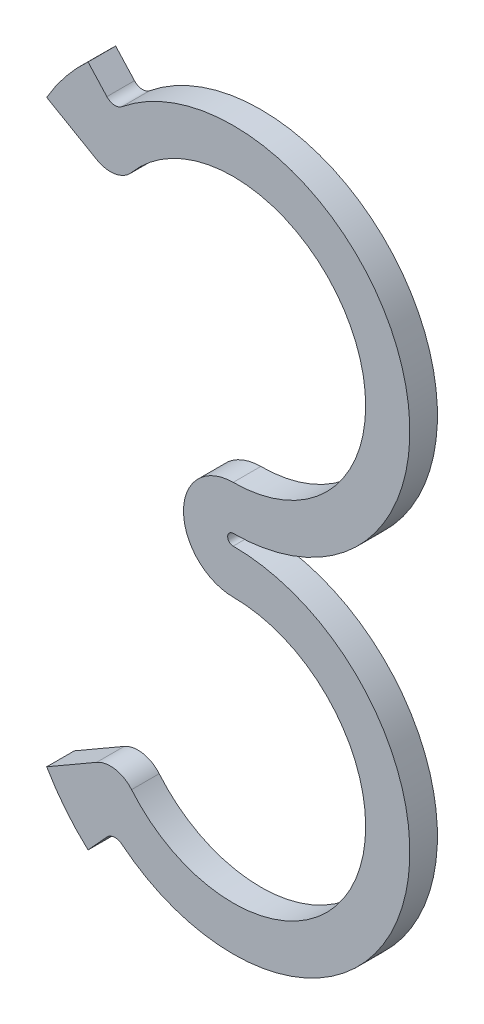
from build123d import *

# Parameters (mm, degrees)
EXTRUDE_1_DEPTH        = 2.5
FILLET_1_R             = 1
FILLET_2_R             = 2.5
FILLET_1_OF_MIRROR_1_R = 1
FILLET_2_OF_MIRROR_1_R = 2.5


with BuildPart() as part:
    # 草图2 → 凸台-拉伸1 (new body)
    with BuildSketch(Plane.XY):
        with BuildLine():
            Line((-4.5, -6.579113924), (-0.5, -6.579113924))
            ThreePointArc((-0.5, -6.579113924), (-0.353553391, -6.225560533), (0, -6.079113924))
            ThreePointArc((0, -6.079113924), (14.918190439, 15.70427557), (-10.784713231, 21.739936821))
            Line((-10.784713231, 21.739936821), (-13.143869251, 24.325354172))
            ThreePointArc((-13.143869251, 24.325354172), (-15.194957506, 22.142312604), (-16.887495374, 19.670886076))
            Line((-16.887495374, 19.670886076), (-10.392304845, 15.920886076))
            ThreePointArc((-10.392304845, 15.920886076), (10.392304845, 15.920886076), (0, -2.079113924))
            ThreePointArc((0, -2.079113924), (-3.181980515, -3.397133409), (-4.5, -6.579113924))
        make_face()
    extrude_1 = extrude(amount=EXTRUDE_1_DEPTH)

    # 圆角1
    fillet_1_edges = [part.edges().sort_by_distance(p)[0] for p in [
        (-10.784713231, 21.739936821, 1.25),
    ]]
    fillet(fillet_1_edges, radius=FILLET_1_R)

    # 圆角2
    fillet_2_edges = [part.edges().sort_by_distance(p)[0] for p in [
        (-10.392304845, 15.920886076, 1.25),
    ]]
    fillet(fillet_2_edges, radius=FILLET_2_R)

    # 镜向1: 凸台-拉伸1 across plane
    add(extrude_1.mirror(Plane.ZX.offset(-6.579113924)))

    # 圆角1 of 镜向1
    fillet_1_of_mirror_1_edges = [part.edges().sort_by_distance(p)[0] for p in [
        (-10.784713231, -34.898164669, 1.25),
    ]]
    fillet(fillet_1_of_mirror_1_edges, radius=FILLET_1_OF_MIRROR_1_R)

    # 圆角2 of 镜向1
    fillet_2_of_mirror_1_edges = [part.edges().sort_by_distance(p)[0] for p in [
        (-10.392304845, -29.079113924, 1.25),
    ]]
    fillet(fillet_2_of_mirror_1_edges, radius=FILLET_2_OF_MIRROR_1_R)


solid = part.part
